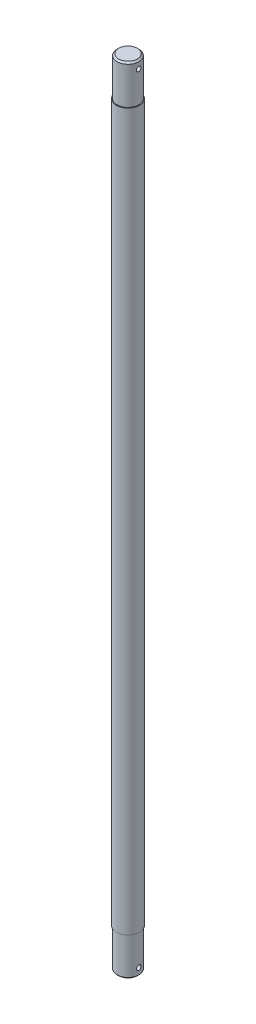
from build123d import *

# Parameters (mm, degrees)
CHAMFER1_SIZE           = 1
CUT_EXTRUDE1_DEPTH      = 511.110282194
CUT_EXTRUDE1_DEPTH_BACK = 511.110282194
SKETCH3_R               = 1.5


with BuildPart() as part:
    # Sketch1 → Revolve1 (revolve)
    with BuildSketch(Plane.XY, mode=Mode.PRIVATE) as revolve1_sk:
        Polygon((0, 0), (7, 0), (7, 25), (7.5, 25), (7.5, 485), (7, 485), (7, 510), (0, 510), align=None)
    revolve(revolve1_sk.sketch.rotate(Axis((0, 0, 0), (0, -1, 0)), 90), axis=Axis((0, 0, 0), (0, -1, 0)))

    # Chamfer1
    chamfer1_edges = [part.edges().sort_by_distance(p)[0] for p in [
        (0, 510, -7),
        (0, 0, -7),
    ]]
    chamfer(chamfer1_edges, length=CHAMFER1_SIZE)

    # Sketch3 → Cut-Extrude1 (cut, two sides: drawn at the far end of the back side and taken through both)
    with BuildSketch(Plane(origin=(0, 0, 0), x_dir=(0, 0, -1), z_dir=(1, 0, 0)).offset(-CUT_EXTRUDE1_DEPTH_BACK)):
        with Locations((0, 505)):
            Circle(SKETCH3_R)
        with Locations((0, 5)):
            Circle(SKETCH3_R)
    extrude(amount=CUT_EXTRUDE1_DEPTH + CUT_EXTRUDE1_DEPTH_BACK, mode=Mode.SUBTRACT)


solid = part.part
